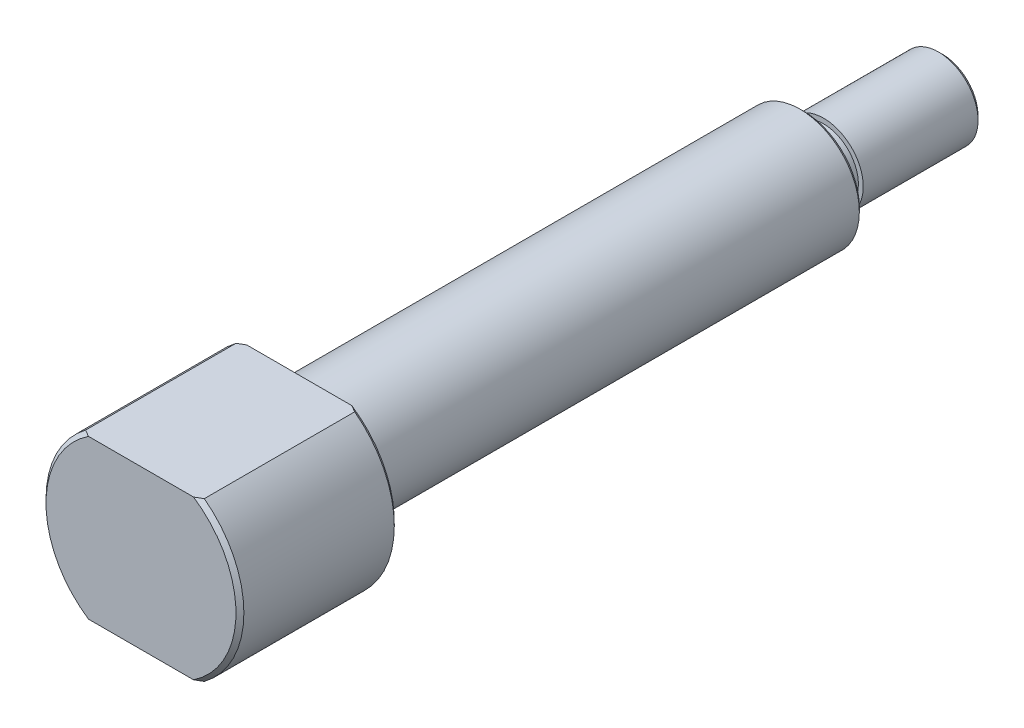
SolidWorks part; units mm, degrees
material "45#"
ref_plane "主视基准图" through (0, 0, 0) normal (0, 0, 1) x (1, 0, 0)
ref_plane "上视基准图" through (0, 0, 0) normal (0, 1, 0) x (1, 0, 0)
ref_plane "右视基准图" through (0, 0, 0) normal (1, 0, 0) x (0, 0, -1)
sketch "草图1" plane through (0, 0, 0) normal (0, 0, 1) x (1, 0, 0)
  circle A0 centre (0, 0) radius 3
  dimension "D1" = 6
extrude "凸台-拉伸1" add sketch "草图1" along normal mid plane 25.5
chamfer "倒角1" distance 0.2 angle 45 1 edges at (3, 0, -12.75)
sketch "草图2" plane through (0, 0, -12.75) normal (0, 0, -1) x (-1, 0, 0)
  circle A0 centre (0, 0) radius 2
  dimension "D1" = 4
extrude "凸台-拉伸2" add sketch "草图2" along normal blind 7
cosmetic thread "装饰螺纹线1" parameters "D1"=6, "D2"=3.242
chamfer "倒角2" distance 0.2 angle 45 1 edges at (-2, 0, -19.75)
sketch "草图3" plane through (0, 0, 12.75) normal (0, 0, 1) x (1, 0, 0)
  circle A0 centre (0, 0) radius 5
  dimension "D1" = 10
extrude "凸台-拉伸3" add sketch "草图3" along normal blind 8
chamfer "倒角3" distance 0.2 angle 45 2 edges at (5, 0, 20.75) (5, 0, 12.75)
sketch "草图4" plane through (0, 0, 20.75) normal (0, 0, 1) x (1, 0, 0)
  line L1 (-15.7364, 10.1363) -> (6.5686, 10.1363)
  line L2 (-15.7364, 10.1363) -> (-15.7364, 4)
  line L3 (-15.7364, 4) -> (6.5686, 4)
  line L4 (6.5686, 10.1363) -> (6.5686, 4)
  line L5 (-15.7364, 10.1363) -> (6.5686, 4) construction
  line L6 (-15.7364, 4) -> (6.5686, 10.1363) construction
  line L7 (18.476, -9.7467) -> (-6.2154, -9.7467)
  line L8 (18.476, -9.7467) -> (18.476, -4)
  line L9 (18.476, -4) -> (-6.2154, -4)
  line L10 (-6.2154, -9.7467) -> (-6.2154, -4)
  line L11 (18.476, -9.7467) -> (-6.2154, -4) construction
  line L12 (18.476, -4) -> (-6.2154, -9.7467) construction
  point P0 (-4.5839, 7.0682)
  point P5 (6.1303, -6.8734)
  dimension "D1" = 8
  dimension "D2" = 4
extrude "切除-拉伸1" cut sketch "草图4" against normal up to surface (8 mm away) up to face at (4.8, 0, 12.75)
sketch "草图5" plane through (0, 0, -12.75) normal (0, 0, -1) x (-1, 0, 0)
  circle A0 centre (0, 0) radius 1.75
  dimension "D1" = 3.5
extrude "切除-拉伸2" cut sketch "草图5" along normal blind 1 flip side to cut
